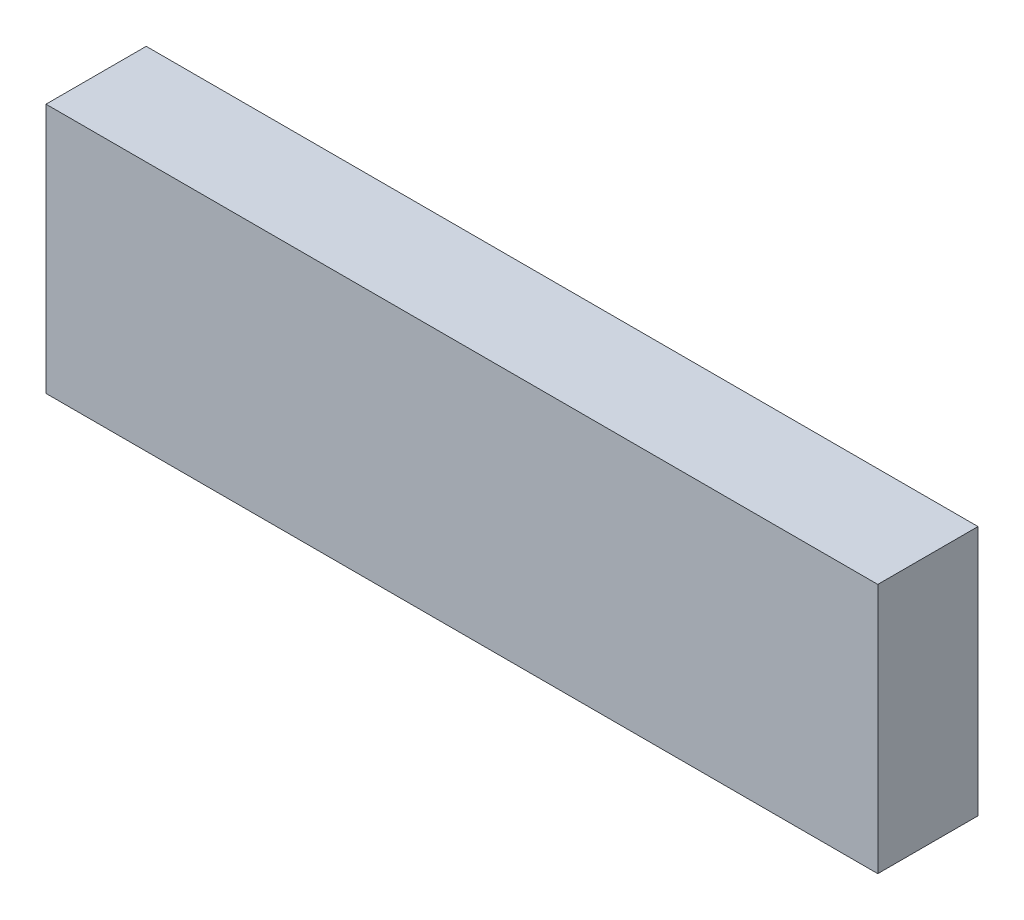
from build123d import *

# Parameters (mm, degrees)
SKETCH1_W           = 166
SKETCH1_H           = 50
BOSS_EXTRUDE1_DEPTH = 20


with BuildPart() as part:
    # Sketch1 → Boss-Extrude1 (new body)
    with BuildSketch(Plane.XY):
        with Locations((83, 25)):
            Rectangle(SKETCH1_W, SKETCH1_H)
    extrude(amount=BOSS_EXTRUDE1_DEPTH)


solid = part.part
